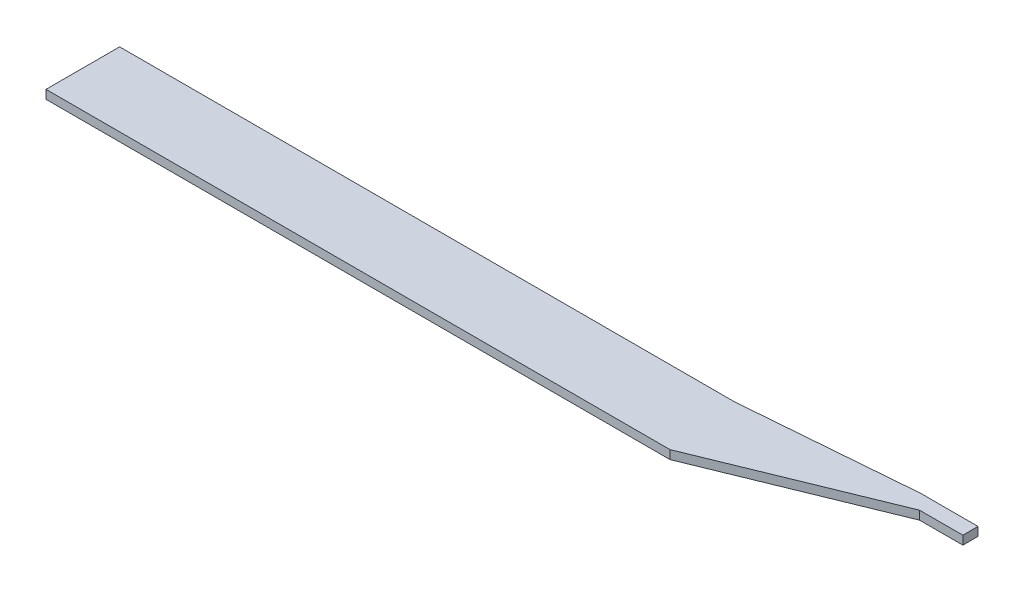
SolidWorks part; units mm, degrees
ref_plane "Front Plane" through (0, 0, 0) normal (0, 0, 1) x (1, 0, 0)
ref_plane "Top Plane" through (0, 0, 0) normal (0, 1, 0) x (1, 0, 0)
ref_plane "Right Plane" through (0, 0, 0) normal (1, 0, 0) x (0, 0, -1)
sketch "Sketch1" plane through (0, 0, 0) normal (0, 1, 0) x (1, 0, 0)
  line L0 (19.5, 1.67) -> (18.5, 1.67)
  line L1 (0, 0) -> (14.4078, 0)
  line L2 (0, 0) -> (0, 1.7)
  line L3 (18.1772, 2.02) -> (19.5, 2.02)
  line L4 (19.5, 1.67) -> (19.5, 2.02)
  line L5 (18.5, 1.67) -> (14.4078, 0)
  line L6 (14.2, 1.7) -> (18.1772, 2.02)
  line L7 (0, 1.7) -> (14.2, 1.7)
  dimension "D1" = 19.5
  dimension "D2" = 2.02
  dimension "D3" = 1.7
  dimension "D4" = 0.35
  dimension "D5" = 22.2
  dimension "D6" = 4.6
  dimension "D7" = 1
  dimension "D8" = 5.3
extrude "Boss-Extrude1" add sketch "Sketch1" along normal blind 0.2
